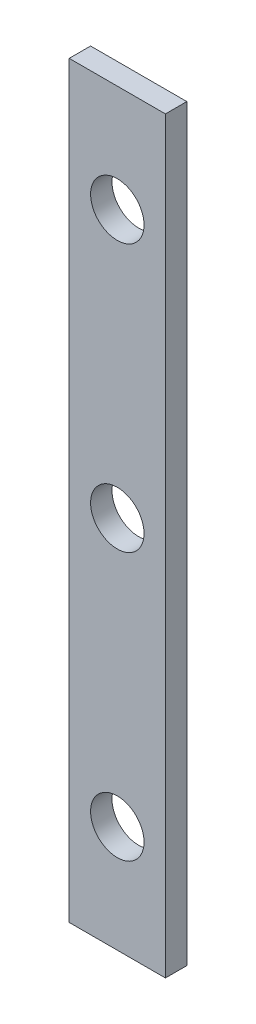
from build123d import *

# Parameters (mm, degrees)
SKETCH_1_W          = 18
SKETCH_1_H          = 140
SKETCH_1_R          = 5
BOSS_EXTRUDE1_DEPTH = 4


with BuildPart() as part:
    # Sketch 1 → Boss-Extrude1 (new body)
    with BuildSketch(Plane.XY):
        Rectangle(SKETCH_1_W, SKETCH_1_H)
        with Locations((0, 50)):
            Circle(SKETCH_1_R, mode=Mode.SUBTRACT)
        Circle(SKETCH_1_R, mode=Mode.SUBTRACT)
        with Locations((0, -50)):
            Circle(SKETCH_1_R, mode=Mode.SUBTRACT)
    extrude(amount=BOSS_EXTRUDE1_DEPTH)


solid = part.part
